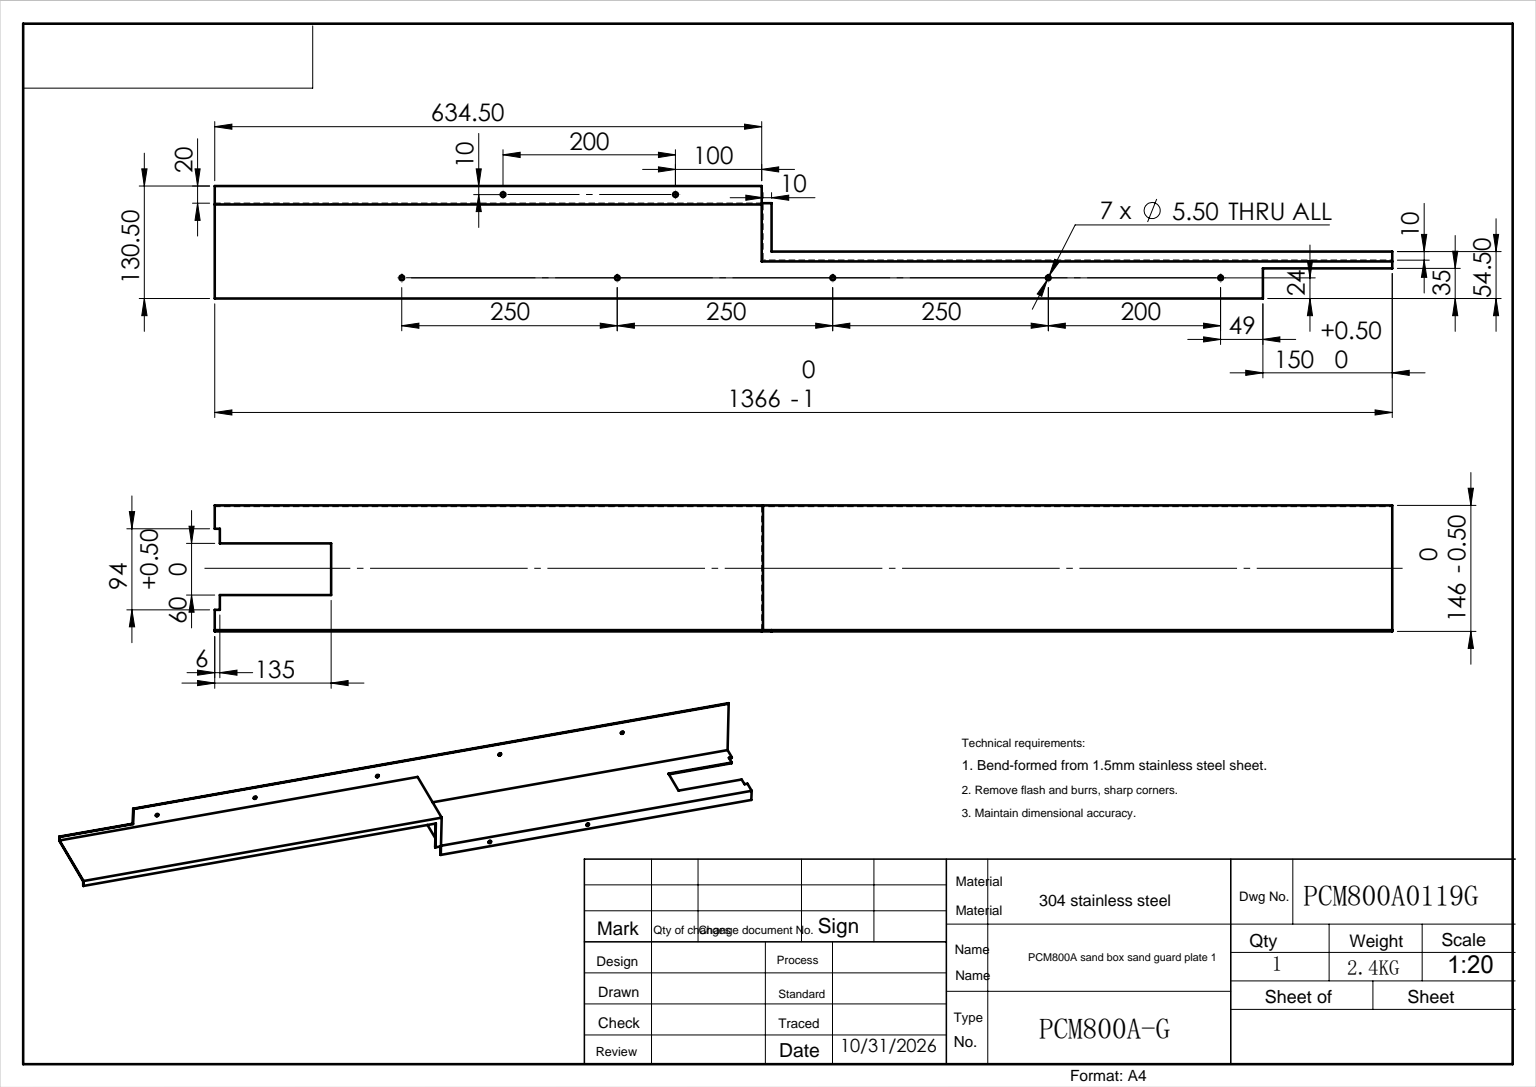
SolidWorks part; units mm, degrees
ref_plane "前视基准面" through (0, 0, 0) normal (0, 0, 1) x (1, 0, 0)
ref_plane "上视基准面" through (0, 0, 0) normal (0, 1, 0) x (1, 0, 0)
ref_plane "右视基准面" through (0, 0, 0) normal (1, 0, 0) x (0, 0, -1)
sketch "草图1" plane through (0, 0, 0) normal (0, 0, 1) x (1, 0, 0)
  line L1 (0, 0) -> (146, 0)
  line L2 (0, 0) -> (0, 636)
  line L3 (0, 636) -> (146, 636)
  line L4 (146, 0) -> (146, 636)
  dimension "D1" = 146
  dimension "D2" = 636
extrude "凸台-拉伸1" add sketch "草图1" along normal blind 1.5
sketch "草图2" plane through (0, 0, 1.5) normal (0, 0, 1) x (1, 0, 0)
  line L0 (0, 0) -> (146, 0) construction
  line L1 (0, 636) -> (1.5, 636)
  line L2 (0, 636) -> (0, 0)
  line L3 (0, 0) -> (1.5, 0)
  line L4 (1.5, 636) -> (1.5, 0)
  dimension "D1" = 1.5
extrude "凸台-拉伸2" add sketch "草图2" along normal blind 109
sketch "草图4" plane through (0, 0, 1.5) normal (0, 0, 1) x (1, 0, 0)
  line L1 (1.5, 0) -> (146, 0)
  line L2 (1.5, 0) -> (1.5, 1.5)
  line L3 (1.5, 1.5) -> (146, 1.5)
  line L4 (146, 0) -> (146, 1.5)
  line L5 (146, 0) -> (146, 636) construction
  dimension "D1" = 1.5
extrude "凸台-拉伸4" add sketch "草图4" along normal blind 66
sketch "草图5" plane through (0, 0, 0) normal (0, -1, 0) x (1, 0, 0)
  line L0 (0, 110.5) -> (0, 66)
  line L1 (0, 110.5) -> (0, 0) construction
  line L2 (0, 66) -> (146, 66)
  line L3 (146, 67.5) -> (146, 0) construction
  line L4 (146, 66) -> (146, 67.5)
  line L5 (146, 67.5) -> (1.5, 67.5)
  line L6 (1.5, 67.5) -> (146, 67.5) construction
  line L7 (1.5, 110.5) -> (1.5, 67.5) construction
  line L8 (1.5, 67.5) -> (1.5, 110.5)
  line L9 (1.5, 110.5) -> (0, 110.5)
  dimension "D1" = 1.5
extrude "凸台-拉伸5" add sketch "草图5" along normal blind 730
sketch "草图6" plane through (0, 0, 0) normal (0, 0, -1) x (-1, 0, 0)
  line L0 (-146, 636) -> (0, 636) construction
  line L1 (-146, 1.5) -> (-144.5, 1.5)
  line L2 (-146, 1.5) -> (-146, 636)
  line L3 (-146, 636) -> (-144.5, 636)
  line L4 (-144.5, 1.5) -> (-144.5, 636)
  line L5 (0, 0) -> (-146, 0) construction
  line L6 (-146, 0) -> (-146, 636) construction
  dimension "D1" = 1.5
  dimension "D2" = 1.5
extrude "凸台-拉伸6" add sketch "草图6" along normal blind 20
sketch "草图7" plane through (0, 0, 66) normal (0, 0, -1) x (-1, 0, 0)
  line L0 (0, -730) -> (-146, -730) construction
  line L1 (-146, 0) -> (-144.5, 0)
  line L2 (-146, 0) -> (-146, -730)
  line L3 (-146, -730) -> (-144.5, -730)
  line L4 (-144.5, 0) -> (-144.5, -730)
  dimension "D1" = 1.5
extrude "凸台-拉伸7" add sketch "草图7" along normal blind 10
sketch "草图8" plane through (0, 0, 0) normal (0, -1, 0) x (1, 0, 0)
  line L1 (144.5, 56) -> (146, 56)
  line L2 (144.5, 56) -> (144.5, 0)
  line L3 (144.5, 0) -> (146, 0)
  line L4 (146, 56) -> (146, 0)
extrude "凸台-拉伸8" add sketch "草图8" along normal blind 10
sketch "草图10" plane through (1.5, 0, 0) normal (1, 0, 0) x (0, 0, -1)
  line L1 (-110.5, -730) -> (-75.5, -730)
  line L2 (-110.5, -730) -> (-110.5, -580)
  line L3 (-110.5, -580) -> (-75.5, -580)
  line L4 (-75.5, -730) -> (-75.5, -580)
  dimension "D1" = 150
  dimension "D2" = 35
extrude "切除-拉伸2" cut sketch "草图10" against normal blind 2
hole_wizard "Ø5.5 (5.5) 直径孔1" positions "草图12" profile "草图11" hole size "Ø5.5" standard "GB" end condition through all
sketch "草图12" plane through (1.5, 0, 0) normal (1, 0, 0) x (0, 0, -1)
  line L0 (-86.5, 636) -> (-86.5, -613.4895) construction
  line L1 (-110.5, 636) -> (-1.5, 636) construction
  line L3 (-110.5, -580) -> (-110.5, 636) construction
  point P1 (-86.5, 419)
  point P3 (-86.5, 169)
  point P5 (-86.5, -81)
  point P7 (-86.5, -331)
  point P9 (-86.5, -531)
  dimension "D1" = 24
  dimension "D2" = 217
  dimension "D3" = 250
  dimension "D4" = 250
  dimension "D5" = 250
  dimension "D6" = 200
sketch "草图11" plane through (1.5, 419, 86.5) normal (0, 1, 0) x (0, 0, -1)
  line L0 (0, 0) -> (0, 1.5001)
  line L1 (0, 1.5001) -> (2.75, 1.5001)
  line L2 (2.75, 1.5001) -> (2.75, 0)
  line L5 (2.75, 0) -> (0, 0)
  line L11 (0, -6.35) -> (0, 107.95) construction
  dimension "通孔孔直径" = 5.5
  dimension "通孔孔深度" = 1.5001
hole_wizard "Ø5.5 (5.5) 直径孔2" positions "草图14" profile "草图13" hole size "Ø5.5" standard "GB"
sketch "草图14" plane through (144.5, 0, 0) normal (-1, 0, 0) x (0, 0, 1)
  line L0 (-10, 1.5) -> (-10, 912.429) construction
  line L1 (-20, 1.5) -> (0, 1.5) construction
  point P0 (-10, 301.5)
  point P1 (-10, 101.5)
  dimension "D1" = 100
  dimension "D2" = 200
sketch "草图13" plane through (144.5, 301.5, -10) normal (0, 1, 0) x (0, 0, 1)
  line L0 (0, 0) -> (0, 3.1524)
  line L1 (0, 3.1524) -> (2.75, 1.5)
  line L2 (2.75, 1.5) -> (2.75, 0)
  line L5 (2.75, 0) -> (0, 0)
  line L10 (0, 3.1524) -> (-2.75, 1.5) construction
  line L11 (0, -6.35) -> (0, 107.95) construction
  dimension "孔直径" = 5.5
  dimension "孔深度" = 1.5
  dimension "导头角度" = 118
sketch "草图15" plane through (0, 0, 1.5) normal (0, 0, 1) x (1, 0, 0)
  line L0 (27, 636) -> (27, 630)
  line L1 (146, 636) -> (1.5, 636) construction
  line L2 (27, 630) -> (44, 630)
  line L3 (44, 630) -> (44, 501)
  line L4 (44, 501) -> (104, 501)
  line L5 (104, 501) -> (104, 630)
  line L6 (104, 630) -> (121, 630)
  line L7 (121, 630) -> (121, 636)
  line L9 (146, 1.5) -> (146, 636) construction
  line L10 (27, 636) -> (121, 636)
  dimension "D1" = 94
  dimension "D2" = 17
  dimension "D3" = 60
  dimension "D4" = 6
  dimension "D5" = 135
  dimension "D6" = 25
  dimension "D7" = 6
extrude "切除-拉伸3" cut sketch "草图15" against normal blind 55
